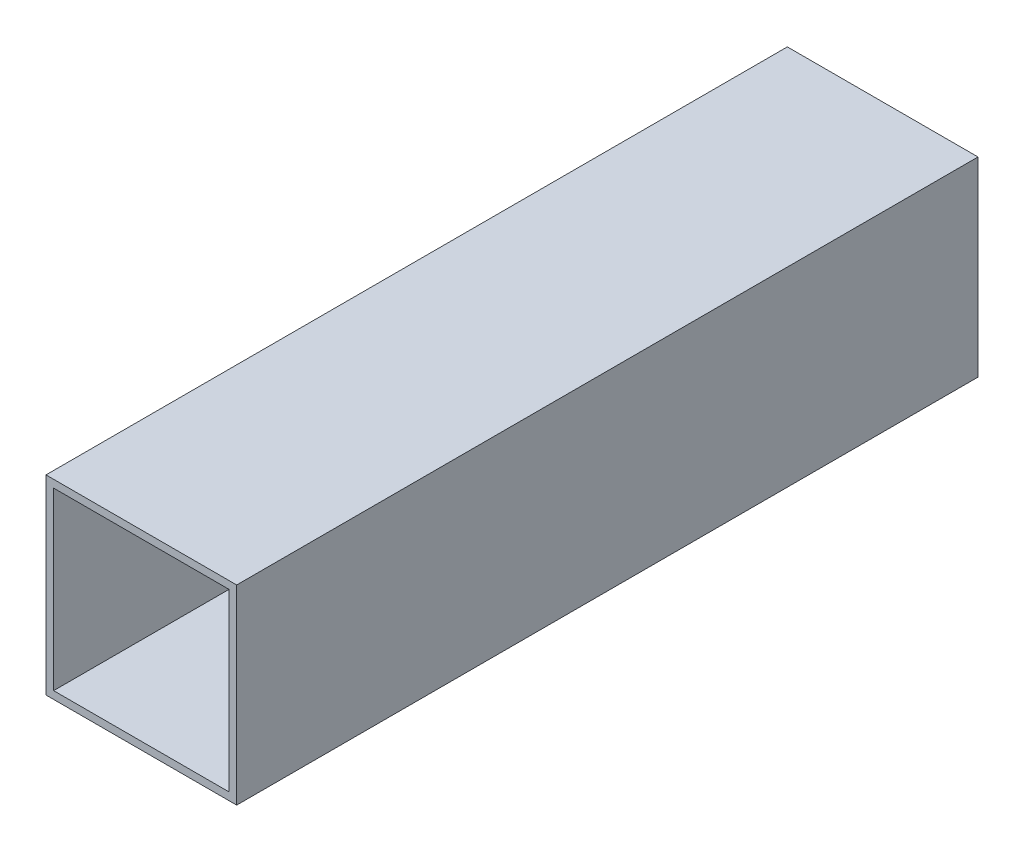
SolidWorks part; units mm, degrees
material "AISI 304"
ref_plane "Front Plane" through (0, 0, 0) normal (0, 0, 1) x (1, 0, 0)
ref_plane "Top Plane" through (0, 0, 0) normal (0, 1, 0) x (1, 0, 0)
ref_plane "Right Plane" through (0, 0, 0) normal (1, 0, 0) x (0, 0, -1)
sketch "Sketch1" plane through (0, 0, 0) normal (0, 0, 1) x (1, 0, 0)
  line L1 (-25, -25) -> (25, -25)
  line L2 (-25, -25) -> (-25, 25)
  line L3 (-25, 25) -> (25, 25)
  line L4 (25, -25) -> (25, 25)
  line L5 (-25, -25) -> (25, 25) construction
  line L6 (-25, 25) -> (25, -25) construction
  line L7 (-23, -23) -> (23, -23)
  line L8 (-23, -23) -> (-23, 23)
  line L9 (-23, 23) -> (23, 23)
  line L10 (23, -23) -> (23, 23)
  line L11 (-23, -23) -> (23, 23) construction
  line L12 (-23, 23) -> (23, -23) construction
  point P0 (0, 0)
  point P6 (0, 0)
  dimension "D1" = 50
  dimension "D2" = 50
  dimension "D3" = 46
  dimension "D4" = 46
extrude "Boss-Extrude1" add sketch "Sketch1" along normal blind 194.4
sketch "Sketch2" plane through (-25, 0, 0) normal (-1, 0, 0) x (0, 0, 1)
  line L0 (97.2, 25) -> (97.2, -132.5751) construction
  line L1 (194.4, 25) -> (0, 25) construction
  line L2 (0, 0) -> (604.8974, 0) construction
  circle A0 centre (36.7, 0) radius 7
  circle A1 centre (157.7, 0) radius 7
  dimension "D1" = 14
  dimension "D2" = 121
extrude "Cut-Extrude1" [suppressed] cut sketch "Sketch2" against normal through all
